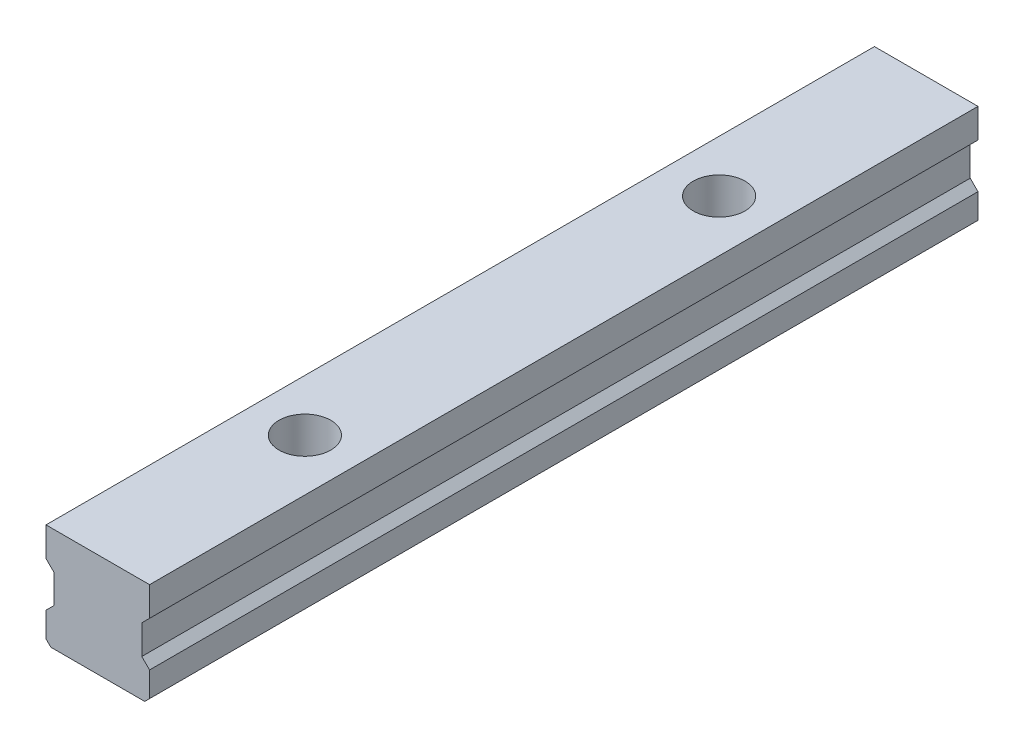
SolidWorks part; units mm, degrees
material "厂家标准"
ref_plane "前视基准面" through (0, 0, 0) normal (0, 0, 1) x (1, 0, 0)
ref_plane "上视基准面" through (0, 0, 0) normal (0, 1, 0) x (1, 0, 0)
ref_plane "右视基准面" through (0, 0, 0) normal (1, 0, 0) x (0, 0, -1)
sketch "草图1" plane through (0, 0, 0) normal (0, 0, 1) x (1, 0, 0)
  line L0 (-7.5, 0) -> (7.5, 0)
  line L1 (-7.5, 0) -> (-7.5, 4.3)
  line L2 (-7.5, 4.3) -> (-6.375, 5.425)
  line L3 (-6.375, 5.425) -> (-6.375, 9.65)
  line L4 (-6.375, 9.65) -> (-7.5, 10.775)
  line L5 (-7.5, 10.775) -> (-7.5, 15)
  line L6 (-7.5, 15) -> (7.5, 15)
  line L7 (0, 0) -> (0, 15) construction
  line L8 (7.5, 10.775) -> (7.5, 15)
  line L9 (6.375, 9.65) -> (7.5, 10.775)
  line L10 (6.375, 5.425) -> (6.375, 9.65)
  line L11 (7.5, 4.3) -> (6.375, 5.425)
  line L12 (7.5, 0) -> (7.5, 4.3)
extrude "凸台-拉伸1" add sketch "草图1" along normal mid plane 100
chamfer "倒角1" distance 0.7 angle 45 2 edges at (7.5, 0, 0) (-7.5, 0, 0)
sketch "草图3" plane through (0, 0, 0) normal (1, 0, 0) x (0, 0, -1)
  line L0 (-30, 15) -> (-30, 0) construction
  line L1 (-50, 15) -> (50, 15) construction
  line L2 (-50, 0) -> (50, 0) construction
  line L3 (-30, 15) -> (-33.75, 15)
  line L4 (-33.75, 15) -> (-33.75, 9.7)
  line L5 (-33.75, 9.7) -> (-32.25, 9.7)
  line L6 (-32.25, 9.7) -> (-32.25, 0)
  line L7 (-32.25, 0) -> (-30, 0)
  line L8 (-30, 15) -> (-30, 18.1542) construction
  line L9 (-30, 0) -> (-30, 15)
  line L10 (-50, 0.7) -> (-50, 4.3) construction
  dimension "E" = 20
  dimension "D沉" = 7.5
  dimension "D通" = 4.5
  dimension "h沉" = 5.3
revolve "上锁孔" cut sketch "草图3" angle 360 about L8
pattern_linear "上锁孔阵列(线性)1" count 2 spacing 60 along (0, 0, -1) of "上锁孔"
other "移动面1" face at (0, 6.55, 50) parameters "D1"=10
other "移动面2" face at (0, 6.55, -50) parameters "D1"=10
equation "\"D2@草图1\"=\"D1@草图1\""
equation "\"D3@草图1\"=\"WR@草图1\"*0.85"
